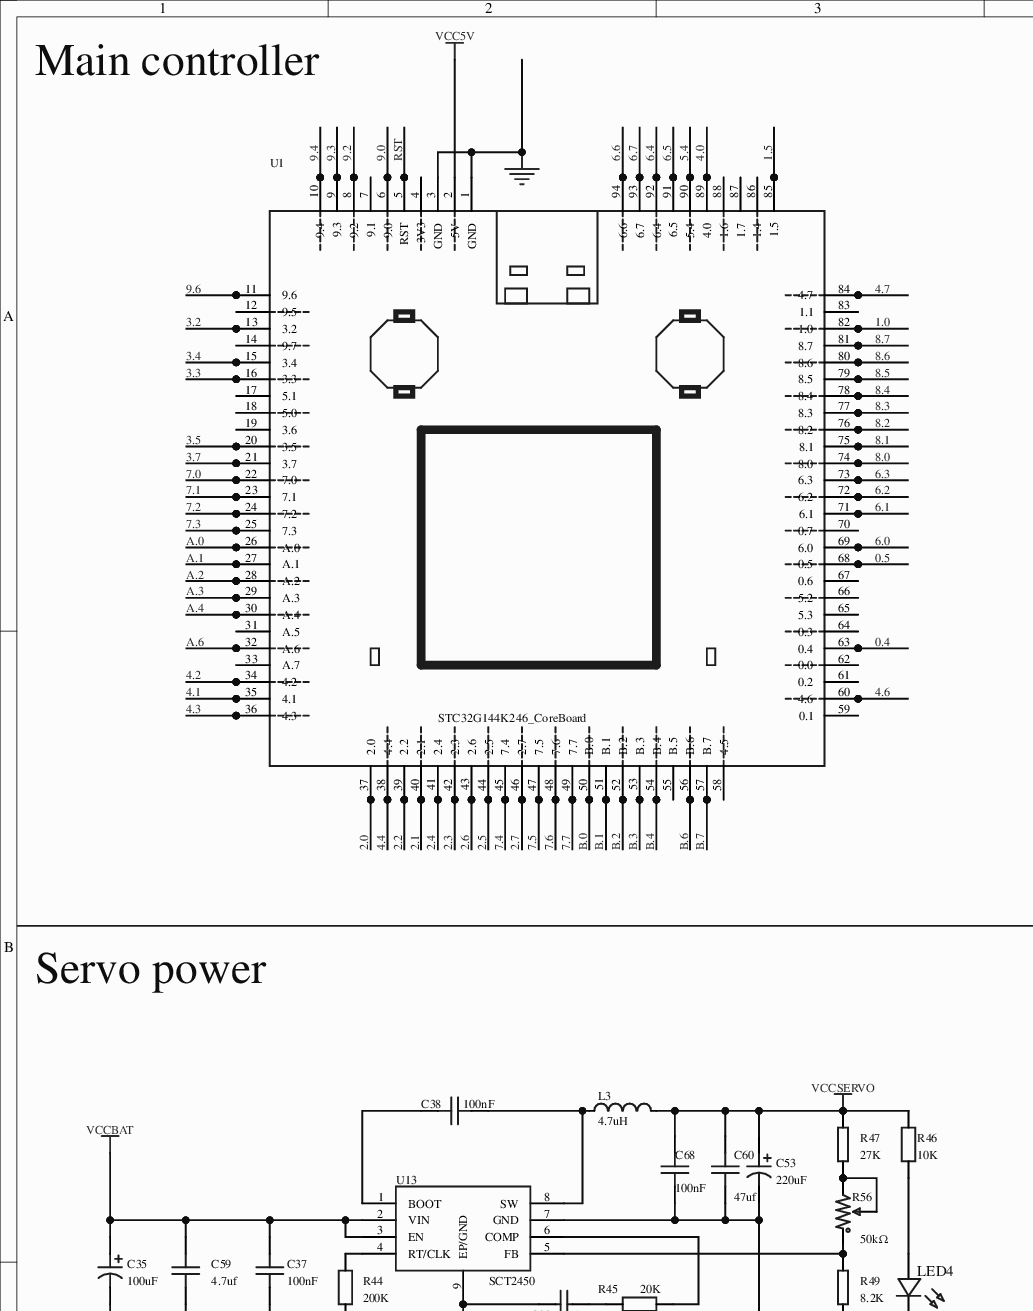
[diagram p0: MISC49918-3.schdoc, top left]
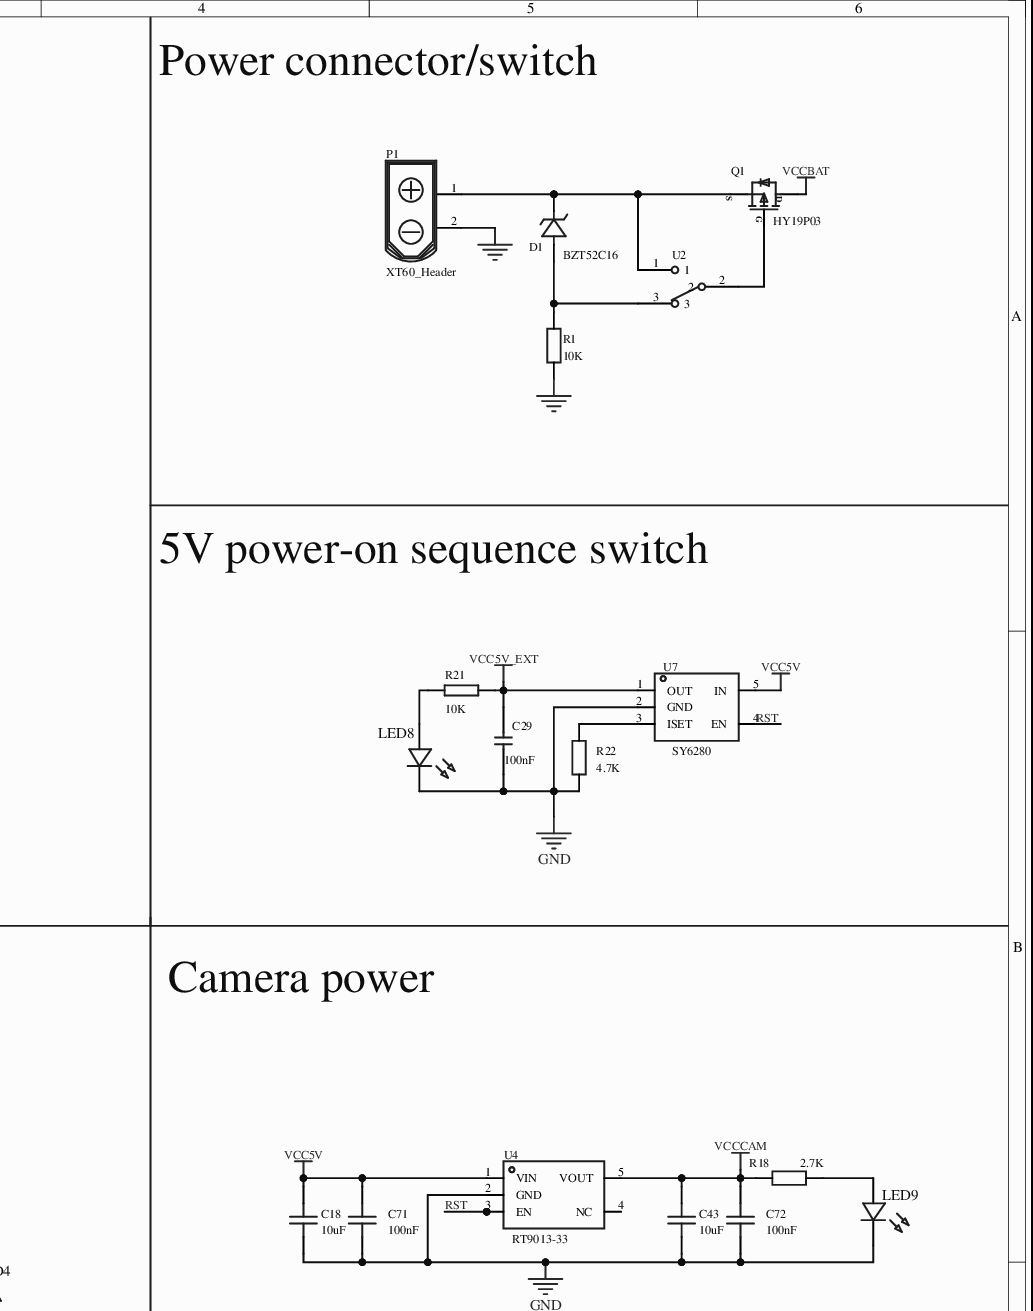
[diagram p1: MISC49918-3.schdoc, top right]
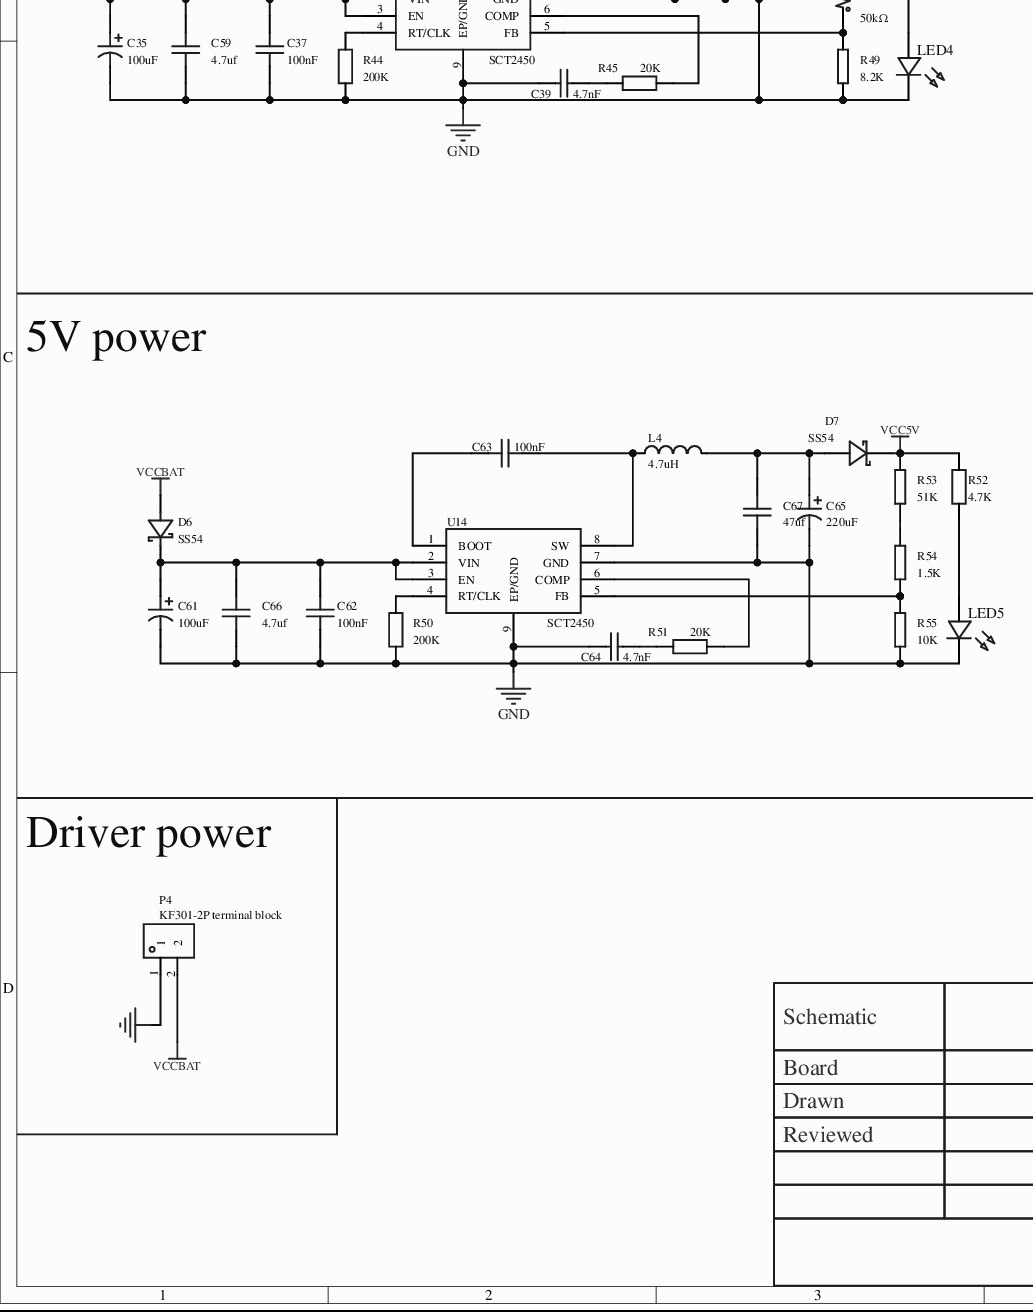
[diagram p2: MISC49918-3.schdoc, bottom left]
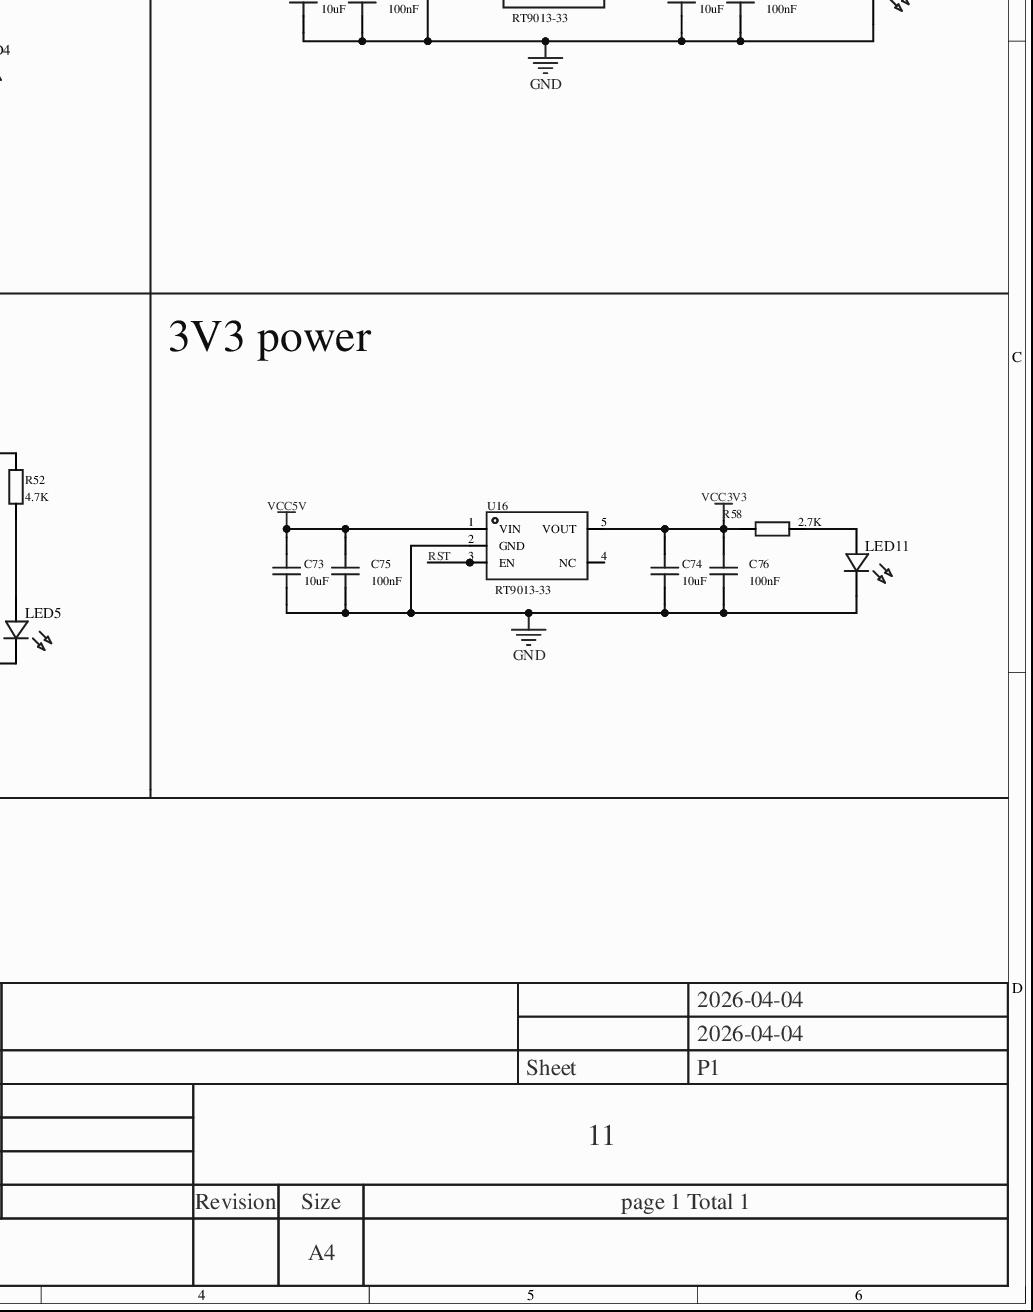
[diagram p3: MISC49918-3.schdoc, bottom right]
# Altium project MISC49918-2.PrjPcb (part 1 of 2)
2 sheets, 130 parts. Net scope: global (net labels, ports and power ports of the same name join across sheets).
Board file: MISC49918.pcbdoc
Sheets:
  MISC49918-3.schdoc
  MISC49918-4.schdoc

## Sheet MISC49918-3.schdoc
size 297 x 381 mm; Version: V1.0; @Project Name: MISC49918; @Update Date: 2026-04-09; @Create Date: 2026-04-09; @Board Name: MISC49918; @Create Time: 13:03:09; @Page Count: 1; @Page No: 1; @Schematic Name: MISC49918; @Update Time: 13:03:09; Size: A4

### Parts
C18  10uF  [C0603]
C29  100nF  [CAPC1608[0603]S-N]
C35  100uF  [CAP-SMD_BD6.3-L6.6-W6.6-LS7.6-FD-1]
C37  100nF  [C0603]
C38  100nF  [C0603]
C39  4.7nF  [C0603]
C43  10uF  [C0603]
C53  220uF  [CAP-SMD_BD6.3-L6.6-W6.6-LS7.6-FD-1]
C59  4.7uf  [C1206]
C60  47uf  [C1206]
C61  100uF  [CAP-SMD_BD6.3-L6.6-W6.6-LS7.6-FD-1]
C62  100nF  [C0603]
C63  100nF  [C0603]
C64  4.7nF  [C0603]
C65  220uF  [CAP-SMD_BD6.3-L6.6-W6.6-LS7.6-FD-1]
C66  4.7uf  [C1206]
C67  47uf  [C1206]
C68  100nF  [C0603]
C71  100nF  [C0603]
C72  100nF  [C0603]
C73  10uF  [C0603]
C74  10uF  [C0603]
C75  100nF  [C0603]
C76  100nF  [C0603]
D1  BZT52C16  [SOD-123_L2.7-W1.6-LS3.7-RD]
D6  SS54  [SMA_L4.3-W2.6-LS5.0-FD]
D7  SS54  [SMA-L[DO-214AC]]
L3  4.7uH  [IND-SMD_L7.2-W6.6_GPSR07X0]
L4  4.7uH  [IND-SMD_L7.2-W6.6_GPSR07X0]
LED4  (no value)  [LED_0603]
LED5  (no value)  [LED_0603]
LED8  (no value)  [LED_0603]
LED9  (no value)  [LED_0603]
LED11  (no value)  [LED_0603]
P1  XT60_Header  [Wired T-Header ThroughHole]
P4  KF301-2P terminal block  [CONN-TH_XY301V-A-5.0-2P]
Q1  HY19P03  [TO-252AA]
R1  10K  [R0603]
R18  2.7K  [R0603]
R21  10K  [RESC1608[0603]S-N]
R22  4.7K  [R0603]
R44  200K  [R0603]
R45  20K  [R0603]
R46  10K  [R0603]
R47  27K  [RESC1608[0603]S-N]
R49  8.2K  [RESC1608[0603]S-N]
R50  200K  [R0603]
R51  20K  [R0603]
R52  4.7K  [R0603]
R53  51K  [RESC1608[0603]S-N]
R54  1.5K  [RESC1608[0603]S-N]
R55  10K  [RESC1608[0603]S-N]
R56  50kΩ  [RES-ADJ-TH_3P-L9.5-W4.85-P2.50-BL-BS]
R58  2.7K  [R0603]
U1  STC32G144K246_CoreBoard  [STC32G144K246_CoreBoard]
U2  (no value)  [SS12D10]
U4  RT9013-33  [SOT-23-5]
U7  SY6280  [SOT-23-5_L3.0-W1.7-P0.95-LS2.8-BL]
U13  SCT2450  [SOP-8E]
U14  SCT2450  [SOP-8E]
U16  RT9013-33  [SOT-23-5]

### Nets
GND: C18.1 C29.1 C35.2 C37.1 C39.1 C43.1 C53.2 C59.1 C60.1 C61.2 C62.1 C64.1 C65.2 C66.1 C67.1 C68.1 C71.1 C72.1 C73.1 C74.1 C75.1 C76.1 LED4.1(C) LED5.1(C) LED8.1(C) LED9.1(C) LED11.1(C) P1.2(-) P4.1 R1.1 R22.1 R44.1 R49.1 R50.1 R55.1 U1.1(GND) U1.3(GND) U4.2(GND) U7.2(GND) U13.7(GND) U13.9(EP/GND) U14.7(GND) U14.9(EP/GND) U16.2(GND)
VCC3V3: C74.2 C76.2 R58.1 U16.5(VOUT)
VCC5V: C18.2 C71.2 C73.2 C75.2 D7.K R52.1 R53.2 U1.2(5V) U4.1(VIN) U7.5(IN) U16.1(VIN)
VCC5V_EXT: C29.2 R21.1 U7.1(OUT)
VCCBAT: C35.1 C37.2 C59.2 D6.1(A) P4.2 Q1.1(D) U13.2(VIN) U13.3(EN)
VCCCAM: C43.2 C72.2 R18.1 U4.5(VOUT)
VCCSERVO: C53.1 C60.2 C68.2 L3.2 R46.1 R47.2
0.4: U1.63(0.4)
0.5: U1.68(0.5)
1.0: U1.82(1.0)
1.5: U1.85(1.5)
2.0: U1.37(2.0)
2.1: U1.40(2.1)
2.2: U1.39(2.2)
2.3: U1.42(2.3)
2.4: U1.41(2.4)
2.5: U1.44(2.5)
2.6: U1.43(2.6)
2.7: U1.46(2.7)
3.2: U1.13(3.2)
3.3: U1.16(3.3)
3.4: U1.15(3.4)
3.5: U1.20(3.5)
3.7: U1.21(3.7)
4.0: U1.89(4.0)
4.1: U1.35(4.1)
4.2: U1.34(4.2)
4.3: U1.36(4.3)
4.4: U1.38(4.4)
4.6: U1.60(4.6)
4.7: U1.84(4.7)
5.4: U1.90(5.4)
6.0: U1.69(6.0)
6.1: U1.71(6.1)
6.2: U1.72(6.2)
6.3: U1.73(6.3)
6.4: U1.92(6.4)
6.5: U1.91(6.5)
6.6: U1.94(6.6)
6.7: U1.93(6.7)
7.0: U1.22(7.0)
7.1: U1.23(7.1)
7.2: U1.24(7.2)
7.3: U1.25(7.3)
7.4: U1.45(7.4)
7.5: U1.47(7.5)
7.6: U1.48(7.6)
7.7: U1.49(7.7)
8.0: U1.74(8.0)
8.1: U1.75(8.1)
8.2: U1.76(8.2)
8.3: U1.77(8.3)
8.4: U1.78(8.4)
8.5: U1.79(8.5)
8.6: U1.80(8.6)
8.7: U1.81(8.7)
9.0: U1.6(9.0)
9.2: U1.8(9.2)
9.3: U1.9(9.3)
9.4: U1.10(9.4)
9.6: U1.11(9.6)
A.0: U1.26(A.0)
A.1: U1.27(A.1)
A.2: U1.28(A.2)
A.3: U1.29(A.3)
A.4: U1.30(A.4)
A.6: U1.32(A.6)
B.0: U1.50(B.0)
B.1: U1.51(B.1)
B.2: U1.52(B.2)
B.3: U1.53(B.3)
B.4: U1.54(B.4)
B.6: U1.56(B.6)
B.7: U1.57(B.7)
RST: U1.5(RST) U4.3(EN) U7.4(EN) U16.3(EN)
NetC38_1: C38.1 L3.1 U13.8(SW)
NetC38_2: C38.2 U13.1(BOOT)
NetC39_2: C39.2 R45.2
NetC61_1: C61.1 C62.2 C66.2 D6.2(K) U14.2(VIN) U14.3(EN)
NetC63_1: C63.1 L4.1 U14.8(SW)
NetC63_2: C63.2 U14.1(BOOT)
NetC64_2: C64.2 R51.2
NetC65_1: C65.1 C67.2 D7.A L4.2
NetD1_1: D1.1(K) P1.1(+) Q1.3(S) U2.1
NetD1_2: D1.2(A) R1.2 U2.3
NetLED4_2: LED4.2(A) R46.2
NetLED5_2: LED5.2(A) R52.2
NetLED8_2: LED8.2(A) R21.2
NetLED9_2: LED9.2(A) R18.2
NetLED11_2: LED11.2(A) R58.2
NetQ1_2: Q1.2(G) U2.2
NetR22_2: R22.2 U7.3(ISET)
NetR44_2: R44.2 U13.4(RT/CLK)
NetR45_1: R45.1 U13.6(COMP)
NetR47_1: R47.1 R56.2 R56.3
NetR49_2: R49.2 R56.1 U13.5(FB)
NetR50_2: R50.2 U14.4(RT/CLK)
NetR51_1: R51.1 U14.6(COMP)
NetR53_1: R53.1 R54.2
NetR54_1: R54.1 R55.2 U14.5(FB)

Not connected (* = marked no-connect by the designer): U1 4(3V3)* 7(9.1)* 12(9.5)* 14(9.7)* 17(5.1)* 18(5.0)* 19(3.6)* 31(A.5)* 33(A.7)* 55(B.5)* 58(4.5)* 59(0.1)* 61(0.2)* 62(0.0)* 64(0.3)* 65(5.3)* 66(5.2)* 67(0.6)* 70(0.7)* 83(1.1)* 86(1.4)* 87(1.7)* 88(1.6)*; U4 4(NC)*; U16 4(NC)*

### Notes on the sheet
- Main controller
- Power connector/switch
- 5V power-on sequence switch
- Servo power
- Camera power
- 5V power
- 3V3 power
- Driver power
- 2026-04-04
- Schematic
- Board
- Sheet
- P1
- Drawn
- Reviewed
- 11
- Revision
- Size
- A4
- page 1 Total 1

### Library data of the parts
C18 C37 C38 C43 C62 C63 C68 C73 C74 = CC0603KRX7R9BB104: Capacitance: 100nF; Tolerance: ±10%; Rated voltage: 50V; Dielectric (temperature coefficient): X7R;; Manufacturer: YAGEO(国巨); 3D Model: ac125912035d415993ca9572d50418b1; 3D Model Transform: 62.992,31.496,0,0,0,0,0,0,0; AddInBom: yes; ModelName: C0603_L1.6-W0.8-H0.8; Device: CC0603KRX7R9BB104; Symbol: CC0603KRX7R9BB104; LCSC Part Name: 100nF ±10% 50V; Supplier Footprint: 0603; Datasheet: https://atta.szlcsc.com/upload/public/pdf/source/20180910/C282072_33301C7F631E79921B82A8DAC6BCC5B3.pdf; Voltage Rated: 50V; Temperature Coefficient: X7R; Supplier: LCSC; Manufacturer Part: CC0603KRX7R9BB104; FootprintName: C0603; ConvertToPcb: yes
  C18 C43 C73 C74: Value: 10uF
  C37 C38 C62 C63 C68: Value: 100nF; Supplier Part: C14663
C29 = 100nF 0603 50V X7R: Voltage: 50V; Type: X7R; Origin Footprint 2: CAPC1608[0603]-L; Origin Footprint 3: CAPC1608[0603]-M; Origin Footprint 4: CAPC1608[0603]-N; Origin Footprint 5: CAPC1608[0603]S-L; Origin Footprint 6: CAPC1608[0603]S-M; AddInBom: yes; Device: 100nF 0603 50V X7R; Symbol: 100nF 0603 50V X7R; Revision: V1.0; Value: 100nF; FootprintName: CAPC1608[0603]S-N; ConvertToPcb: yes
C35 C53 C61 C65 = RVE100UF35V67RV0072: Capacitance: 100uF; Tolerance: ±20%; Rated voltage: 35V; Ripple current: 230mA@120Hz; ESR: 600mΩ@100kHz;; Manufacturer: KNSCHA(科尼盛); 3D Model: e9bf03a505e14561b78f20847edc0c03; 3D Model Transform: 283.464,259.842,0,180,0,0,0,0,0; φD: 6.3mm; L: 7.7mm; Lifetime @ Temp: 2000hrs@105℃; AddInBom: yes; Device: RVE100UF35V67RV0072; Symbol: RVE100UF35V67RV0072; LCSC Part Name: 100uF ±20% 35V; Manufacturer Part: RVE100UF35V67RV0072; Supplier Footprint: SMD,D6.3xL7.7mm; Datasheet: https://atta.szlcsc.com/upload/public/pdf/source/20220719/B52EB46F8A1558448ED03D8B4CB3C24F.pdf; Supplier: LCSC; Rated Voltage: 35V; Ripple Current: 230mA@120Hz; Equivalent Series Resistance(ESR): 600mΩ@100kHz; Operating Temperature: -55℃~+105℃; FootprintName: CAP-SMD_BD6.3-L6.6-W6.6-LS7.6-FD-1; ConvertToPcb: yes; ModelName: CAP-SMD_BD6.3-L6.6-W6.6-LS7.6-FD-1
  C35 C61: Supplier Part: C2836437; Value: 100uF
  C53 C65: Value: 220uF
C39 C64 = 0603B472K500NT: Capacitance: 4.7nF; Tolerance: ±10%; Rated voltage: 50V; Dielectric (temperature coefficient): X7R;; Manufacturer: FH(风华); 3D Model: ac125912035d415993ca9572d50418b1; 3D Model Transform: 62.992,31.496,0,0,0,0,0,0,0; AddInBom: yes; ModelName: C0603_L1.6-W0.8-H0.8; Device: 0603B472K500NT; Symbol: 0603B472K500NT; LCSC Part Name: 4.7nF ±10% 50V; Supplier Part: C53987; Manufacturer Part: 0603B472K500NT; Supplier Footprint: 0603; Datasheet: https://atta.szlcsc.com/upload/public/pdf/source/20200305/C486355_26A10D38EF8C2A5C37091D0039909270.pdf; Supplier: LCSC; Value: 4.7nF; Voltage Rated: 50V; Temperature Coefficient: X7R; FootprintName: C0603; ConvertToPcb: yes
C59 C60 C66 C67 = CAP_1206: Symbol: Capacitance; 3D Model: e4be705b945545a48e666415e3682bd8; 3D Model Transform: 125.984,62.992,0,0,0,0,0,0,0; ConvertToPcb: yes; ModelName: C1206_L3.2-W1.6-H1.3; Device: CAP_1206; Supplier Footprint: 1206; FootprintName: C1206; AddInBom: yes
  C59 C66: Value: 4.7uf
  C60 C67: Value: 47uf
C71 C72 C75 C76 = CAP_0603: Symbol: Capacitance; 3D Model: ac125912035d415993ca9572d50418b1; 3D Model Transform: 62.992,31.496,0,0,0,0,0,0,0; ConvertToPcb: yes; ModelName: C0603_L1.6-W0.8-H0.8; Device: CAP_0603; Supplier Footprint: 0603; Value: 100nF; FootprintName: C0603; AddInBom: yes
D1 = BZT52C16: Zener voltage (nominal): -; Power: 500mW; Tolerance: -;; Manufacturer: Slkor(萨科微); Symbol: BZT52C16_C707145; 3D Model: ad7e39f9e5534b3c96ffdc5532ebb493; 3D Model Transform: 146.026,62.992,0,180,0,0,0.0005,0,0; Reverse Leakage Current (Ir): 100nA@11.2V; AddInBom: yes; ModelName: SOD-123_L2.7-W1.6-H1.4-LS3.7; Device: BZT52C16; LCSC Part Name: BZT52C16; Supplier Footprint: SOD-123; Datasheet: https://atta.szlcsc.com/upload/public/pdf/source/20200721/C707125_BAEA70ACC1B0F60BBAC1FD71D8806D24.pdf; Zener Voltage (Nom): -; Power Dissipation: 500mW; Tolerance: -; Supplier: LCSC; Supplier Part: C707145; Manufacturer Part: BZT52C16; JLCPCB Part Class: Extended library; FootprintName: SOD-123_L2.7-W1.6-LS3.7-RD; ConvertToPcb: yes
D6 = SS54_C7420369: Diode configuration: single; Forward voltage (Vf): 550mV@5.0A; DC reverse voltage (Vr): 40V; Average rectified current (Io): 5A;; Manufacturer: 宏迦橙; 3D Model: 7e24bebe6cd74171ae8c9de6fc5b78aa; 3D Model Transform: 198.4248,103.5431,0,180,0,0,0,0,0; Reverse Leakage Current (Ir): 50uA@40V; Peak forward surge current: 120A; AddInBom: yes; Device: SS54_C7420369; Symbol: SS54_C7420369; LCSC Part Name: 电压:40V 电流:5A; Supplier Footprint: SMA(DO-214AC); Datasheet: https://atta.szlcsc.com/upload/public/pdf/source/20230828/254C3882F8647358AD9F60DD73611B5E.pdf; Diode Configuration: Single; Forward Voltage (Vf@If): 550mV@5.0A; Reverse Voltage (Vr): 40V; Average Rectified Current (Io): 5A; Supplier: LCSC; Supplier Part: C7420369; Manufacturer Part: SS54; FootprintName: SMA_L4.3-W2.6-LS5.0-FD; ConvertToPcb: yes; ModelName: SMA_L4.3-W2.6-LS5.0-FD
D7 = SS54: AddInBom: yes; Device: SS54; Symbol: SS54; Revision: V1.0; Value: SS54; FootprintName: SMA-L[DO-214AC]; ConvertToPcb: yes
L3 L4 = CYA0630-4.7UH: Inductance: 4.7uH; Tolerance: ±20%; Rated current: 5A; DC resistance (DCR): 34.5mΩ;; Manufacturer: SHOU HAN(首韩); 3D Model: 21a538e04f2f4eba8e6ad942a7c3dde1; 3D Model Transform: 283.464,259.842,0,0,0,0,0.003,0,0; AddInBom: yes; ModelName: IND-SMD_L7.2-W6.6-H3.0_GPSR07X0; Device: CYA0630-4.7UH; Symbol: CYA0630-4.7UH; LCSC Part Name: 4.7uH ±20%; Supplier Footprint: SMD,7.2x6.6mm; Datasheet: https://atta.szlcsc.com/upload/public/pdf/source/20221010/79ACBE86DD414F23A670753564343C1B.pdf; Rated Current: 5A; DC Resistance (DCR): 34.5mΩ; Supplier: LCSC; Supplier Part: C5189748; Manufacturer Part: CYA0630-4.7UH; Value: 4.7uH; FootprintName: IND-SMD_L7.2-W6.6_GPSR07X0; ConvertToPcb: yes
LED4 LED5 LED8 LED9 LED11 = LED_0603-R: Symbol: LED_R; Convert to PCB: yes; 3D Model: dd8257b0d61a4cd7b68939a056e08095; 3D Model Transform: 58.72,29.4,22.03,0,0,0,0,0,0; ModelName: LED-0603_R; Device: LED_0603-R; Add into BOM: yes; Supplier Footprint: 0603; FootprintName: LED_0603
P1 = XT60_Header: Origin Footprint 2: XT60UM; Origin Footprint 3: Wired T-Header; Origin Footprint 4: XT60UF; AddInBom: yes; Device: XT60_Header; Symbol: XT60_Header; FootprintName: Wired T-Header ThroughHole; ConvertToPcb: yes
P4 = KF301-2P接线端子: Manufacturer: null; Add into BOM: yes; Contributor: lcsc; ModelId: ef7ead88b0f2448d904975b26718870f; ModelTransform: 0,0,0,0,0,0,0,0,0; Device: KF301-2P terminal block; Symbol: KF301-2P terminal block; Convert to PCB: yes; Origin Footprint: CONN-TH_XY301V-A-5.0-2P; Supplier: LCSC; Supplier Part: C9900016950; JLCPCB Part Class: Extended Part; spicePre: P; spiceSymbolName: KF301-2P terminal block; FootprintName: CONN-TH_XY301V-A-5.0-2P; ModelName: CONN-TH_XY301V-A-5.0-2P
Q1 = HY19P03: AddInBom: yes; Device: HY19P03; Symbol: HY19P03; FootprintName: TO-252AA; ConvertToPcb: yes
R1 R18 R22 R44-R46 R50-R52 R58 = Res_0603: Symbol: Resistor; 3D Model: fc143cca1e79419f9cd78b61e9279f08; 3D Model Transform: 31.8897,63.7794,0,90,0,0,0,0,0; ConvertToPcb: yes; Device: Res_0603; Supplier Footprint: 0603; FootprintName: R0603; AddInBom: yes; ModelName: R0603
  R1 R46: Value: 10K
  R18 R58: Value: 2.7K
  R22 R52: Value: 4.7K
  R44 R50: Value: 200K
  R45 R51: Value: 20K
R21 R49 R55 = Res-Chip: Tolerance: ±1%; Origin Footprint 2: RESC0603[0201]-L; Origin Footprint 3: RESC0603[0201]-M; Origin Footprint 4: RESC0603[0201]-N; Origin Footprint 5: RESC0603[0201]S-L; Origin Footprint 6: RESC0603[0201]S-M; Origin Footprint 7: RESC0603[0201]S-N; Origin Footprint 8: RESC1005[0402]-L; Origin Footprint 9: RESC1005[0402]-M; Origin Footprint 10: RESC1005[0402]-N; Origin Footprint 11: RESC1005[0402]S-L; Origin Footprint 12: RESC1005[0402]S-M; Origin Footprint 13: RESC1005[0402]S-N; Origin Footprint 14: RESC1608[0603]-L; Origin Footprint 15: RESC1608[0603]-M; Origin Footprint 16: RESC1608[0603]-N; Origin Footprint 17: RESC1608[0603]S-L; Origin Footprint 18: RESC1608[0603]S-M; Origin Footprint 19: RESC2012[0805]; Origin Footprint 20: RESC2012[0805]S-L; Origin Footprint 21: RESC2012[0805]S-M; Origin Footprint 22: RESC2012[0805]S-N; Origin Footprint 23: RESC3216[1206]; Origin Footprint 24: RESC3216[1206]S-L; Origin Footprint 25: RESC3216[1206]S-M; Origin Footprint 26: RESC3216[1206]S-N; Origin Footprint 27: RESC3225[1210]; Origin Footprint 28: RESC3225[1210]S; Origin Footprint 29: RESC5025[2010]; Origin Footprint 30: RESC5025[2010]S; Origin Footprint 31: RESC6332[2512]; Origin Footprint 32: RESC6332[2512]S; Origin Footprint 33: RESC0402[01005]-L; AddInBom: yes; Device: Res-Chip; Symbol: Res-Chip; Revision: V1.0; FootprintName: RESC1608[0603]S-N; ConvertToPcb: yes
  R21 R55: Value: 10K
  R49: Value: 8.2K
R47 R53 = Res-Chip_6: Tolerance: ±1%; Origin Footprint 2: RESC0603[0201]-L; Origin Footprint 3: RESC0603[0201]-M; Origin Footprint 4: RESC0603[0201]-N; Origin Footprint 5: RESC0603[0201]S-L; Origin Footprint 6: RESC0603[0201]S-M; Origin Footprint 7: RESC0603[0201]S-N; Origin Footprint 8: RESC1005[0402]-L; Origin Footprint 9: RESC1005[0402]-M; Origin Footprint 10: RESC1005[0402]-N; Origin Footprint 11: RESC1005[0402]S-L; Origin Footprint 12: RESC1005[0402]S-M; Origin Footprint 13: RESC1005[0402]S-N; Origin Footprint 14: RESC1608[0603]-L; Origin Footprint 15: RESC1608[0603]-M; Origin Footprint 16: RESC1608[0603]-N; Origin Footprint 17: RESC1608[0603]S-L; Origin Footprint 18: RESC1608[0603]S-M; Origin Footprint 19: RESC2012[0805]; Origin Footprint 20: RESC2012[0805]S-L; Origin Footprint 21: RESC2012[0805]S-M; Origin Footprint 22: RESC2012[0805]S-N; Origin Footprint 23: RESC3216[1206]; Origin Footprint 24: RESC3216[1206]S-L; Origin Footprint 25: RESC3216[1206]S-M; Origin Footprint 26: RESC3216[1206]S-N; Origin Footprint 27: RESC3225[1210]; Origin Footprint 28: RESC3225[1210]S; Origin Footprint 29: RESC5025[2010]; Origin Footprint 30: RESC5025[2010]S; Origin Footprint 31: RESC6332[2512]; Origin Footprint 32: RESC6332[2512]S; Origin Footprint 33: RESC0402[01005]-L; AddInBom: yes; Device: Res-Chip_6; Symbol: Res-Chip_6; Revision: V1.0; FootprintName: RESC1608[0603]S-N; ConvertToPcb: yes
  R47: Value: 27K
  R53: Value: 51K
R54 = Res-Chip_7: Tolerance: ±1%; Origin Footprint 2: RESC0603[0201]-L; Origin Footprint 3: RESC0603[0201]-M; Origin Footprint 4: RESC0603[0201]-N; Origin Footprint 5: RESC0603[0201]S-L; Origin Footprint 6: RESC0603[0201]S-M; Origin Footprint 7: RESC0603[0201]S-N; Origin Footprint 8: RESC1005[0402]-L; Origin Footprint 9: RESC1005[0402]-M; Origin Footprint 10: RESC1005[0402]-N; Origin Footprint 11: RESC1005[0402]S-L; Origin Footprint 12: RESC1005[0402]S-M; Origin Footprint 13: RESC1005[0402]S-N; Origin Footprint 14: RESC1608[0603]-L; Origin Footprint 15: RESC1608[0603]-M; Origin Footprint 16: RESC1608[0603]-N; Origin Footprint 17: RESC1608[0603]S-L; Origin Footprint 18: RESC1608[0603]S-M; Origin Footprint 19: RESC2012[0805]; Origin Footprint 20: RESC2012[0805]S-L; Origin Footprint 21: RESC2012[0805]S-M; Origin Footprint 22: RESC2012[0805]S-N; Origin Footprint 23: RESC3216[1206]; Origin Footprint 24: RESC3216[1206]S-L; Origin Footprint 25: RESC3216[1206]S-M; Origin Footprint 26: RESC3216[1206]S-N; Origin Footprint 27: RESC3225[1210]; Origin Footprint 28: RESC3225[1210]S; Origin Footprint 29: RESC5025[2010]; Origin Footprint 30: RESC5025[2010]S; Origin Footprint 31: RESC6332[2512]; Origin Footprint 32: RESC6332[2512]S; Origin Footprint 33: RESC0402[01005]-L; AddInBom: yes; Device: Res-Chip_7; Symbol: Res-Chip_7; Revision: V1.0; Value: 1.5K; FootprintName: RESC1608[0603]S-N; ConvertToPcb: yes
R56 = 3296W-1-503_C48997928: Resistance: 50kΩ; Tolerance: ±10%; Power: 500mW; Temperature coefficient: ±250ppm/℃;; Manufacturer: JIERR(捷而瑞); 3D Model: b182808559bb43bda9e7de64b64134cb; 3D Model Transform: 374.015,188.976,0,90,0,0,0,0,-137.795; Number of Turns: 28; AddInBom: yes; ModelName: 3296W; Device: 3296W-1-503_C48997928; Symbol: 3296W-1-503_C48997928; LCSC Part Name: 3296W-1-503; Supplier Part: C48997928; Manufacturer Part: 3296W-1-503; Supplier Footprint: 插件-3P,9.5x4.9mm; JLCPCB Part Class: Extended library; Datasheet: https://item.szlcsc.com/datasheet/3296W-1-503/51342064.html; Supplier: LCSC; Value: 50kΩ; Power(Watts): 500mW; Temperature Coefficient: ±250ppm/℃; FootprintName: RES-ADJ-TH_3P-L9.5-W4.85-P2.50-BL-BS; ConvertToPcb: yes
U1 = STC32G144K246_CoreBoard: STC32G144K246_Core Seekfree STC32G144K246 core board; componentDisplayMode: -1; AddInBom: yes; Device: STC32G144K246_CoreBoard; Symbol: STC32G144K246_CoreBoard; Footprint Name: STC32G144K246_CoreBoard; ConvertToPcb: yes
U2 = kaiguan: AddInBom: yes; Device: kaiguan; Symbol: kaiguan; FootprintName: SS12D10; ConvertToPcb: yes
U4 U16 = RT9013-33GU5: Output type: fixed; Max input voltage: 5.5V; Output voltage: 3.3V; Max output current: 500mA; Power supply rejection ratio (PSRR): 50dB@(10kHz); Output polarity: positive;; Manufacturer: RICHTEK(立锜); 3D Model: 722cd094cbf94024931010e5fd938fc2; 3D Model Transform: 82.677,78.74,0,0,0,0,0,0,0; Dropout Voltage: 400mV@(500mA); standby current: 50uA; Number of Outputs: 1; AddInBom: yes; ModelName: SC-70-5_L2.0-W1.3-P0.65-LS2.1-BR; Device: RT9013-33GU5; Symbol: RT9013-33GU5; Manufacturer Part: RT9013-33; LCSC Part Name: RT9013-33GU5; Supplier Part: C3034127; Supplier Footprint: SC-70-5; Datasheet: https://atta.szlcsc.com/upload/public/pdf/source/20220613/DD4CF7EAF1F9097C51D5D7DB1A8622BA.pdf; Supplier: LCSC; Output Type: Fixed; Maximum Input Voltage: 5.5V; Output Voltage: 3.3V; MAX Output Current: 500mA; Power Supply Rejection Ratio (PSRR): 50dB@(10kHz); Operating Temperature: -40℃~+85℃; Output Polarity: Positive; FootprintName: SOT-23-5; ConvertToPcb: yes
U7 = SY6280AAC_C55136: Low-power distribution switch; Manufacturer: silergy(矽力杰); 3D Model: 0a2a1b8f50944f73965918ad6e5fe167; 3D Model Transform: 118.60433,114.173,0,90,0,0,0.0005,0.0005,0; AddInBom: yes; ModelName: SOT-23-5_L2.9-W1.6-H1.1-LS2.8-P0.95; Device: SY6280AAC_C55136; Symbol: SY6280AAC; Manufacturer Part: SY6280; LCSC Part Name: SY6280AAC; Supplier Part: C55136; Supplier Footprint: SOT-23-5; Datasheet: https://atta.szlcsc.com/upload/public/pdf/source/20161108/1478586372822.pdf; Supplier: LCSC; FootprintName: SOT-23-5_L3.0-W1.7-P0.95-LS2.8-BL; ConvertToPcb: yes
U13 U14 = SCT2450: AddInBom: yes; Device: SCT2450; Symbol: SCT2450; FootprintName: SOP-8E; ConvertToPcb: yes